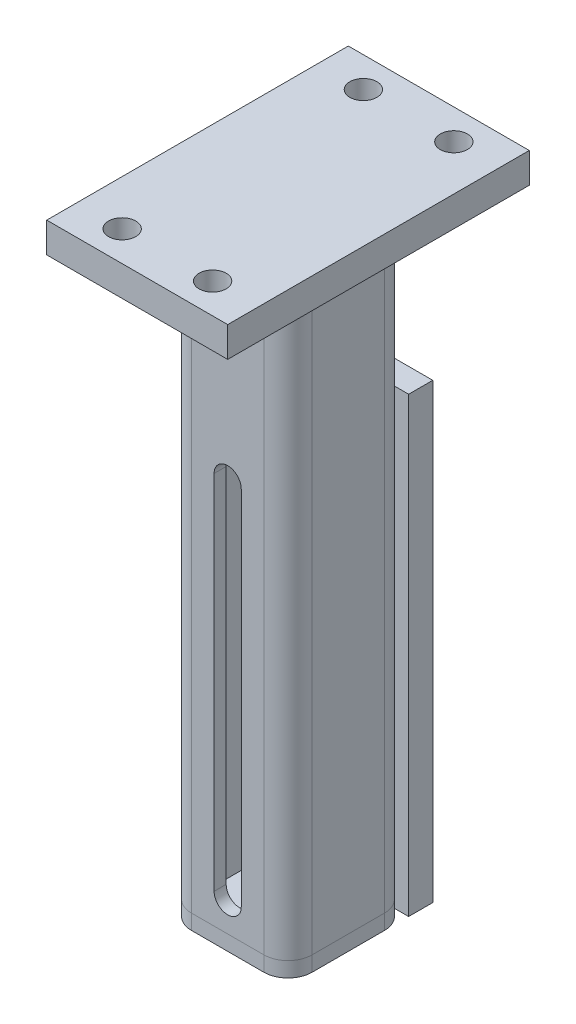
SolidWorks part; units mm, degrees
ref_plane "前视基准面" through (0, 0, 0) normal (0, 0, 1) x (1, 0, 0)
ref_plane "上视基准面" through (0, 0, 0) normal (0, 1, 0) x (1, 0, 0)
ref_plane "右视基准面" through (0, 0, 0) normal (1, 0, 0) x (0, 0, -1)
sketch "草图2" plane through (0, 0, 0) normal (0, 0, 1) x (1, 0, 0)
  line L0 (0, 0) -> (0, 200)
  dimension "D1" = 200
other "方管 40 X 40 X 4.0(1)"
ref_plane "基准面1" through (0, 0, 0) normal (0, 1, 0) x (-1, 0, 0)
sketch "Sketch1" plane through (0, 0, 0) normal (0, 1, 0) x (-1, 0, 0)
  line L0 (-12, -16) -> (12, -16)
  line L1 (-16, -12) -> (-16, 12)
  line L2 (12, 16) -> (-12, 16)
  line L3 (16, 12) -> (16, -12)
  line L4 (-12, -20) -> (12, -20)
  line L5 (-20, -12) -> (-20, 12)
  line L6 (12, 20) -> (-12, 20)
  line L7 (20, 12) -> (20, -12)
  line L8 (-20, 0) -> (-16, 0) construction
  line L9 (-16, 0) -> (16, 0) construction
  line L10 (16, 0) -> (20, 0) construction
  line L12 (0, 20) -> (0, 16) construction
  line L13 (0, 16) -> (0, -16) construction
  line L14 (0, -16) -> (0, -20) construction
  arc A0 (20, 12) -> (12, 20) centre (12, 12) ccw
  arc A1 (12, -20) -> (20, -12) centre (12, -12) ccw
  arc A2 (-20, -12) -> (-12, -20) centre (-12, -12) ccw
  arc A3 (-12, 20) -> (-20, 12) centre (-12, 12) ccw
  arc A4 (-12, 16) -> (-16, 12) centre (-12, 12) ccw
  arc A5 (16, 12) -> (12, 16) centre (12, 12) ccw
  arc A6 (12, -16) -> (16, -12) centre (12, -12) ccw
  arc A7 (-16, -12) -> (-12, -16) centre (-12, -12) ccw
  point P2 (-20, 20)
  point P33 (-20, -20)
  point P34 (20, -20)
  point P36 (20, 20)
  point P37 (0, 0)
  dimension "D1" = 8
  dimension "Thickness" = 4
  dimension "V_leg" = 40
  dimension "H_leg" = 40
sketch "草图4" plane through (0, 200, 0) normal (0, 1, 0) x (1, 0, 0)
  line L1 (-30, 50) -> (30, 50)
  line L2 (-30, 50) -> (-30, -50)
  line L3 (-30, -50) -> (30, -50)
  line L4 (30, 50) -> (30, -50)
  line L5 (-30, 50) -> (30, -50) construction
  line L6 (-30, -50) -> (30, 50) construction
  point P0 (0, 0)
  dimension "D1" = 100
  dimension "D2" = 60
extrude "凸台-拉伸1" add sketch "草图4" along normal blind 10 separate body
other "顶端盖1" parameters "D1"=5, "D2"=3, "D3"=8, "D4"=0
hole_wizard "Ø9.0 (9) 直径孔1" positions "草图5" profile "草图6" hole size "Ø9.0" standard "GB" end condition through all
sketch "草图5" plane through (0, 200, 0) normal (0, -1, 0) x (-1, 0, 0)
  line L0 (0, 50) -> (0, -58.9494) construction
  line L1 (-30, 50) -> (30, 50) construction
  line L3 (-20, 0) -> (52.1373, 0) construction
  line L4 (-20, 12) -> (-20, -12) construction
  point P0 (-15, 40)
  point P2 (15, 40)
  point P4 (-15, -40)
  point P6 (15, -40)
  dimension "D1" = 30
  dimension "D2" = 80
sketch "草图6" plane through (15, 200, -40) normal (1, 0, 0) x (0, 0, -1)
  line L0 (0, 0) -> (0, 10)
  line L1 (0, 10) -> (4.5, 10)
  line L2 (4.5, 10) -> (4.5, 0)
  line L5 (4.5, 0) -> (0, 0)
  line L11 (0, -6.35) -> (0, 107.95) construction
  dimension "通孔孔直径" = 9
  dimension "通孔孔深度" = 10
sketch "草图8" plane through (0, 0, -20) normal (0, 0, -1) x (-1, 0, 0)
  line L0 (20, 200) -> (20, 5) construction
  line L1 (-20, 0) -> (20, 0)
  line L2 (-20, 0) -> (-20, 150)
  line L3 (-20, 150) -> (20, 150)
  line L4 (20, 0) -> (20, 150)
  dimension "D1" = 150
extrude "凸台-拉伸2" add sketch "草图8" along normal blind 8 separate body
sketch "草图9" plane through (0, 0, -28) normal (0, 0, -1) x (-1, 0, 0)
  line L0 (0, 135) -> (0, 15) construction
  line L1 (0, 0) -> (0, 200) construction
  line L2 (4.5, 135) -> (4.5, 15)
  line L3 (-4.5, 135) -> (-4.5, 15)
  arc A0 (4.5, 135) -> (-4.5, 135) centre (0, 135) ccw
  arc A1 (-4.5, 15) -> (4.5, 15) centre (0, 15) ccw
  point P4 (0, 75)
  dimension "D1" = 9
  dimension "D2" = 120
  dimension "D3" = 15
extrude "切除-拉伸1" cut sketch "草图9" against normal through all
